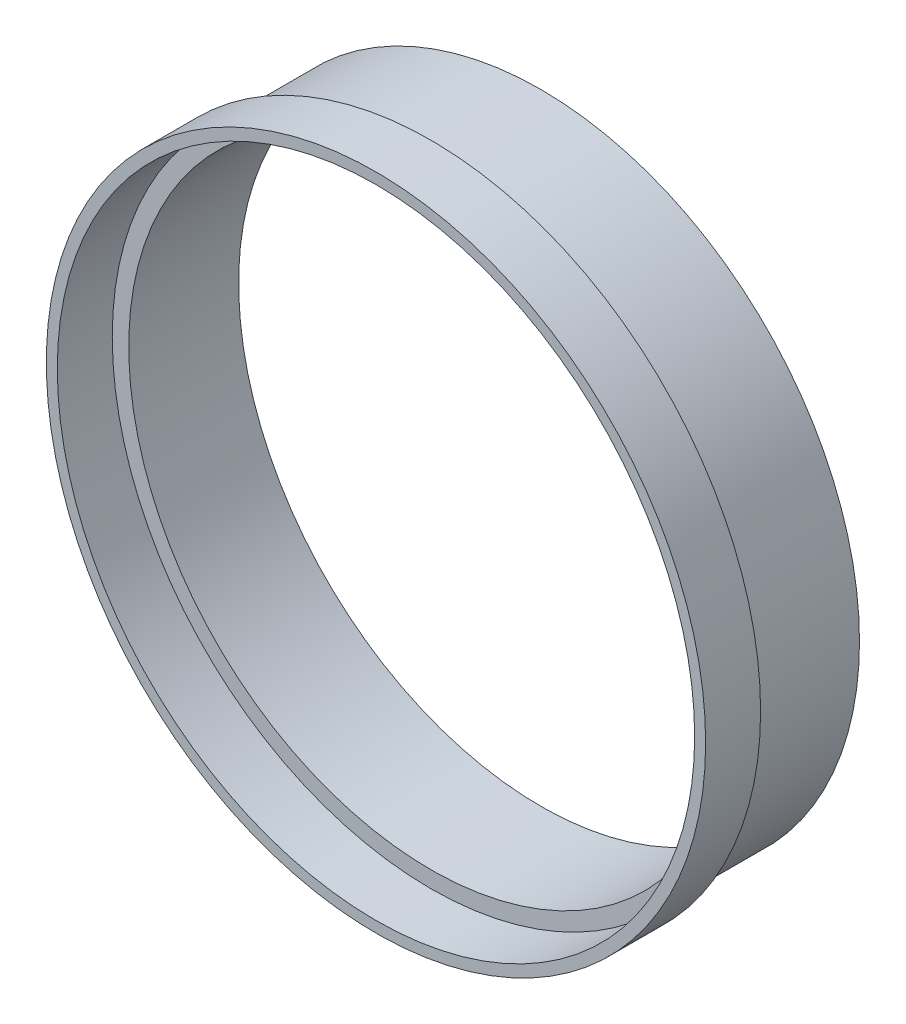
from build123d import *

# Parameters (mm, degrees)
SKETCH1_R           = 58
SKETCH1_R_2         = 55
BOSS_EXTRUDE1_DEPTH = 20
SKETCH2_R           = 60
SKETCH2_R_2         = 58
BOSS_EXTRUDE2_DEPTH = 10


with BuildPart() as part:
    # Sketch1 → Boss-Extrude1 (new body)
    with BuildSketch(Plane.XY):
        Circle(SKETCH1_R)
        Circle(SKETCH1_R_2, mode=Mode.SUBTRACT)
    extrude(amount=BOSS_EXTRUDE1_DEPTH)


with BuildPart() as body_2:
    # Sketch2 → Boss-Extrude2 (new body)
    with BuildSketch(Plane.XY.offset(20)):
        Circle(SKETCH2_R)
        Circle(SKETCH2_R_2, mode=Mode.SUBTRACT)
    extrude(amount=BOSS_EXTRUDE2_DEPTH)


solid = Compound([part.part, body_2.part])
